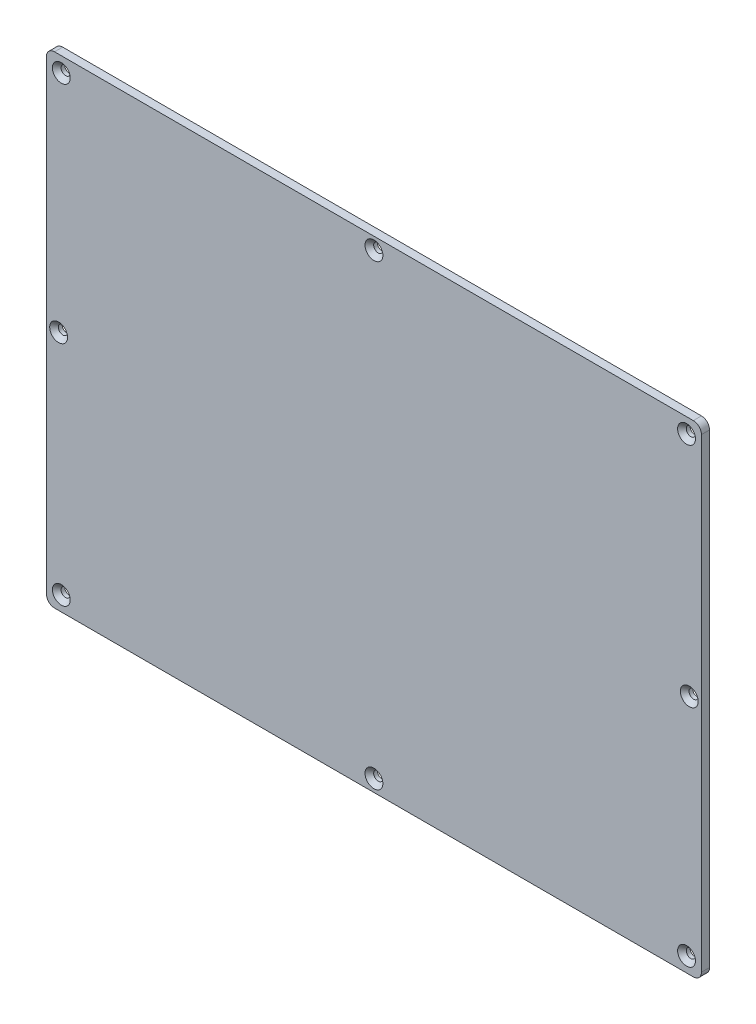
from build123d import *

# Parameters (mm, degrees)
SKETCH1_W                                         = 242
SKETCH1_H                                         = 178
BOSS_EXTRUDE1_DEPTH                               = 3
FILLET1_R                                         = 3
HOLE_SIZE_PER_CROSS_FOR_HALF_COUNTERS_D           = 3.4
HOLE_SIZE_PER_CROSS_FOR_HALF_COUNTERS_DEPTH       = 20
HOLE_SIZE_PER_CROSS_FOR_HALF_COUNTERS_CSINK_D     = 6.6
HOLE_SIZE_PER_CROSS_FOR_HALF_COUNTERS_CSINK_ANGLE = 90
HOLE_SIZE_PER_CROSS_FOR_HALF_COUNTERS_TIP         = 1.021463052


with BuildPart() as part:
    # Sketch1 → Boss-Extrude1 (new body)
    with BuildSketch(Plane.XY):
        Rectangle(SKETCH1_W, SKETCH1_H)
    extrude(amount=BOSS_EXTRUDE1_DEPTH)

    # Fillet1
    fillet1_edges = [part.edges().sort_by_distance(p)[0] for p in [
        (121, -89, 1.5),
        (-121, -89, 1.5),
        (-121, 89, 1.5),
        (121, 89, 1.5),
    ]]
    fillet(fillet1_edges, radius=FILLET1_R)

    # Hole size (% per cross) for half-countersunk slotted wood screw, type 1
    with Locations(Plane.XY.offset(3)):
        with Locations((0, 84.5), (-116.5, 0), (0, -84.5), (116.5, 0), (-115.5, 83.5), (-115.5, -83.5), (115.5, -83.5), (115.5, 83.5)):
            CounterSinkHole(HOLE_SIZE_PER_CROSS_FOR_HALF_COUNTERS_D / 2, HOLE_SIZE_PER_CROSS_FOR_HALF_COUNTERS_CSINK_D / 2, depth=HOLE_SIZE_PER_CROSS_FOR_HALF_COUNTERS_DEPTH, counter_sink_angle=HOLE_SIZE_PER_CROSS_FOR_HALF_COUNTERS_CSINK_ANGLE)
            with Locations((0, 0, -(HOLE_SIZE_PER_CROSS_FOR_HALF_COUNTERS_DEPTH + HOLE_SIZE_PER_CROSS_FOR_HALF_COUNTERS_TIP / 2))):  # 118° drill point
                Cone(0, HOLE_SIZE_PER_CROSS_FOR_HALF_COUNTERS_D / 2, HOLE_SIZE_PER_CROSS_FOR_HALF_COUNTERS_TIP, mode=Mode.SUBTRACT)


solid = part.part
